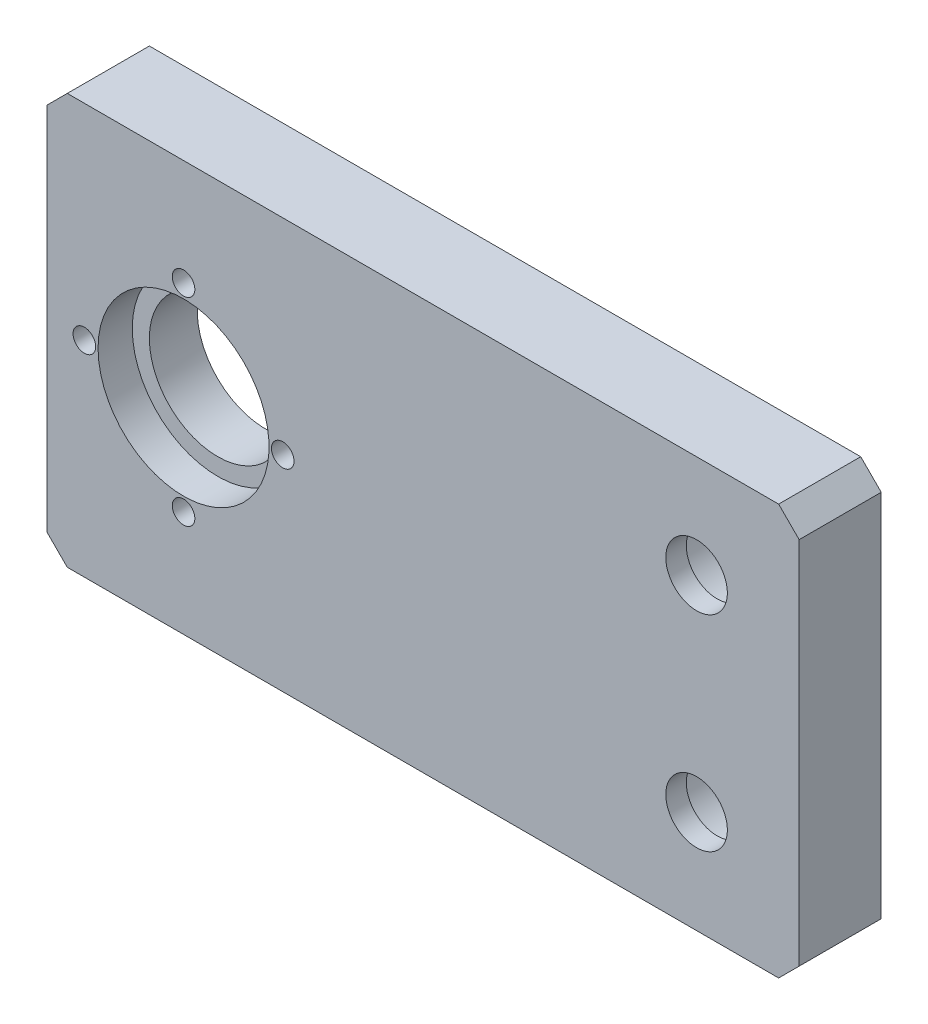
SolidWorks part; units mm, degrees
ref_plane "Front Plane" through (0, 0, 0) normal (0, 0, 1) x (1, 0, 0)
ref_plane "Top Plane" through (0, 0, 0) normal (0, 1, 0) x (1, 0, 0)
ref_plane "Right Plane" through (0, 0, 0) normal (1, 0, 0) x (0, 0, -1)
sketch "Sketch1" plane through (0, 0, 0) normal (0, 0, 1) x (1, 0, 0)
  line L1 (-55, -30) -> (55, -30)
  line L2 (-55, -30) -> (-55, 30)
  line L3 (-55, 30) -> (55, 30)
  line L4 (55, -30) -> (55, 30)
  line L5 (-55, -30) -> (55, 30) construction
  line L6 (-55, 30) -> (55, -30) construction
  point P0 (0, 0)
  dimension "D1" = 60
  dimension "D2" = 110
extrude "Boss-Extrude1" add sketch "Sketch1" along normal blind 12
sketch "Sketch2" plane through (0, 0, 12) normal (0, 0, -1) x (-1, 0, 0)
  line L1 (55, 30) -> (55, -30) construction
  line L2 (55, 0) -> (35, 0) construction
  circle A0 centre (35, 0) radius 12.5
  dimension "D1" = 25
  dimension "D2" = 20
extrude "Cut-Extrude1" cut sketch "Sketch2" along normal blind 5
sketch "Sketch3" plane through (0, 0, 12) normal (0, 0, 1) x (1, 0, 0)
  circle A0 centre (-35, 0) radius 10
  dimension "D1" = 20
extrude "Cut-Extrude3" cut sketch "Sketch3" against normal through all
chamfer "Chamfer1" distance 3 angle 45 4 edges at (-55, -30, 6) (-55, 30, 6) (55, 30, 6) (55, -30, 6)
hole_wizard "M4 Tapped Hole1" positions "Sketch4" profile "Sketch5" tap size "M4" standard "GB" end condition through all
sketch "Sketch4" plane through (0, 0, 12) normal (0, 0, 1) x (1, 0, 0)
  line L0 (0, 0) -> (-55, 0) construction
  line L1 (-55, 27) -> (-55, -27) construction
  line L3 (-35, 0) -> (-35, 14.5) construction
  point P0 (-35, 14.5)
  point P13 (-20.5, 0)
  point P16 (-49.5, 0)
  point P17 (-35, -14.5)
  dimension "D1" = 14.5
  dimension "D2" = 20
  dimension "D3" = 34.5
sketch "Sketch5" plane through (-35, 14.5, 12) normal (1, 0, 0) x (0, -1, 0)
  line L0 (0, 0) -> (0, 12)
  line L1 (0, 12) -> (1.65, 12)
  line L2 (1.65, 12) -> (1.65, 0)
  line L5 (1.65, 0) -> (0, 0)
  line L11 (0, -6.35) -> (0, 107.95) construction
  dimension "通孔螺纹孔钻头直径" = 3.3
  dimension "通孔螺纹孔钻头深度" = 12
cosmetic thread "Hole thread line1" parameters "D2"=4
cosmetic thread "Hole thread line2" parameters "D2"=4
cosmetic thread "Hole thread line3" parameters "D2"=4
cosmetic thread "Hole thread line4" parameters "D2"=4
hole_wizard "CBORE for M8 Hexagon socket head cap screws1" positions "Sketch8" profile "Sketch9" counterbore size "M8" standard "GB" end condition through all
sketch "Sketch8" plane through (0, 0, 0) normal (0, 0, -1) x (-1, 0, 0)
  line L0 (-55, -27) -> (-55, 27) construction
  line L1 (-52, 30) -> (52, 30) construction
  point P13 (-40, 15)
  point P15 (-40, -15)
  dimension "D1" = 15
  dimension "D2" = 15
  dimension "D3" = 30
sketch "Sketch9" plane through (40, 15, 0) normal (1, 0, 0) x (0, 1, 0)
  line L0 (0, 0) -> (0, 12)
  line L1 (0, 12) -> (4.5, 12)
  line L3 (4.5, 12) -> (4.5, 9)
  line L4 (4.5, 9) -> (7.5, 9)
  line L5 (7.5, 9) -> (7.5, 0)
  line L7 (7.5, 0) -> (0, 0)
  line L11 (0, -6.35) -> (0, 107.95) construction
  dimension "通孔孔直径" = 9
  dimension "通孔孔深度" = 12
  dimension "柱形沉头孔直径" = 15
  dimension "柱形沉头孔深度" = 9
equation "\"1\"= \"代号代号\""
equation "\"2\"= \"名称代号\""
